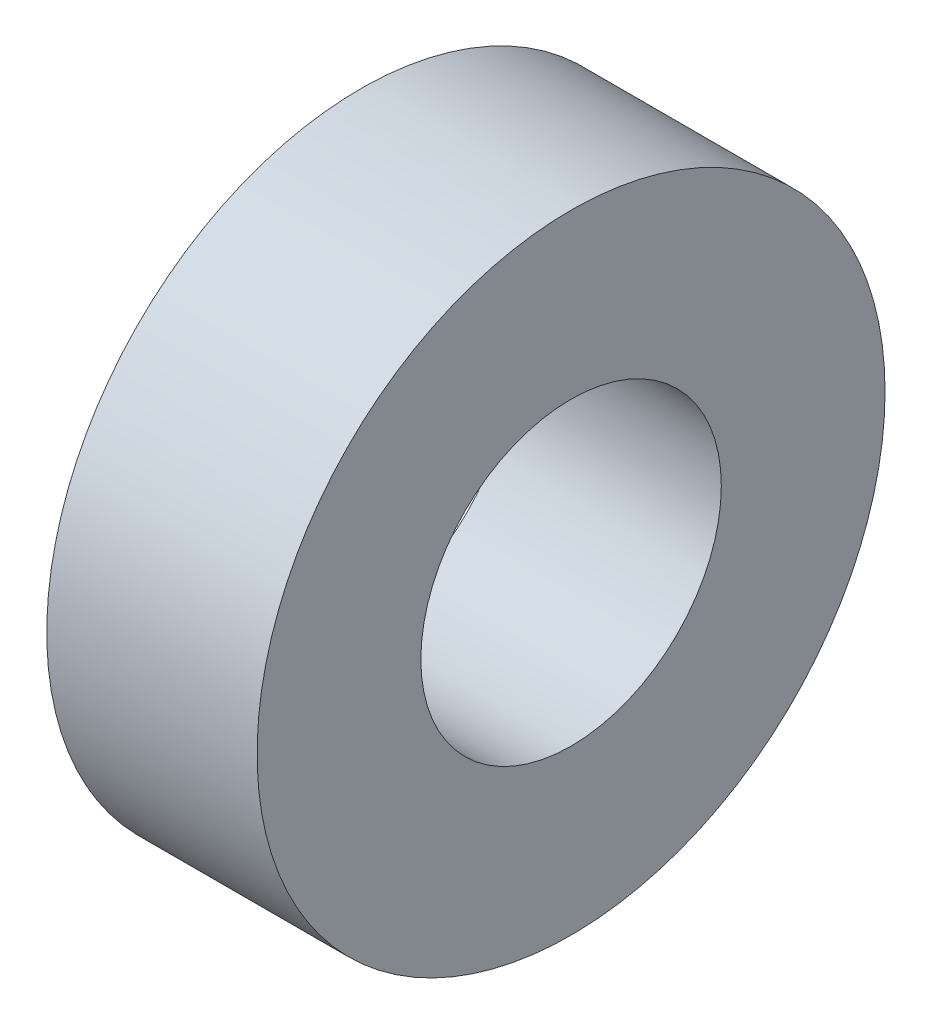
from build123d import *

# Parameters (mm, degrees)
SKETCH_1_R      = 41.8
SKETCH_1_R_2    = 20
EXTRUDE_1_DEPTH = 28


with BuildPart() as part:
    # 草图1 → 凸台-拉伸1 (new body)
    with BuildSketch(Plane(origin=(0, 0, 0), x_dir=(0, 0, -1), z_dir=(1, 0, 0))):
        Circle(SKETCH_1_R)
        Circle(SKETCH_1_R_2, mode=Mode.SUBTRACT)
    extrude(amount=EXTRUDE_1_DEPTH)


solid = part.part
